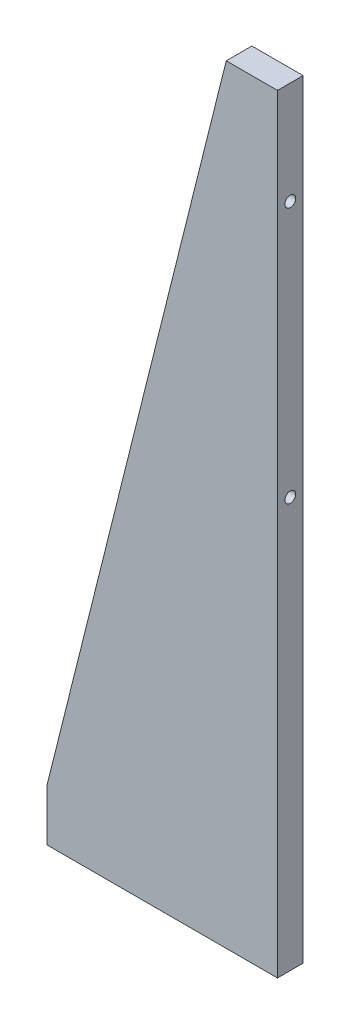
from build123d import *

# Parameters (mm, degrees)
SKETCH_1_W             = 90
SKETCH_1_H             = 300
EXTRUDE_1_DEPTH        = 10
CUT_EXTRUDE_1_REACH    = 158.924
HOLE_WIZARD_M5_1_D     = 4.2
HOLE_WIZARD_M5_1_DEPTH = 14.4
HOLE_WIZARD_M5_1_TIP   = 1.2618073
HOLE_WIZARD_M5_2_D     = 4.2
HOLE_WIZARD_M5_2_DEPTH = 14.4
HOLE_WIZARD_M5_2_TIP   = 1.2618073


with BuildPart() as part:
    # 草图1 → 凸台-拉伸1 (new body)
    with BuildSketch(Plane.XY):
        Rectangle(SKETCH_1_W, SKETCH_1_H)
    extrude(amount=EXTRUDE_1_DEPTH)

    # 草图2 → 切除-拉伸1 (cut, up to next)
    with BuildSketch(Plane.XY.offset(10), mode=Mode.PRIVATE) as cut_extrude_1_sk1:
        Polygon((25, 150), (-45, 150), (-45, -130), align=None)
    cut_extrude_1_tool1 = extrude(cut_extrude_1_sk1.sketch, amount=-CUT_EXTRUDE_1_REACH, mode=Mode.PRIVATE) & part.part
    add(cut_extrude_1_tool1.solids().sort_by_distance((-21.666667, 56.666667, 10))[0], mode=Mode.SUBTRACT)

    # M5 螺纹孔1
    with Locations(Plane(origin=(0, -150, 0), x_dir=(-1, 0, 0), z_dir=(0, -1, 0))):
        with Locations((-25, -5), (25, -5)):
            Hole(HOLE_WIZARD_M5_1_D / 2, depth=HOLE_WIZARD_M5_1_DEPTH)
            with Locations((0, 0, -(HOLE_WIZARD_M5_1_DEPTH + HOLE_WIZARD_M5_1_TIP / 2))):  # 118° drill point
                Cone(0, HOLE_WIZARD_M5_1_D / 2, HOLE_WIZARD_M5_1_TIP, mode=Mode.SUBTRACT)

    # M5 螺纹孔2
    with Locations(Plane(origin=(45, 0, 0), x_dir=(0, 0, -1), z_dir=(1, 0, 0))):
        with Locations((-5, 110), (-5, 10)):
            Hole(HOLE_WIZARD_M5_2_D / 2, depth=HOLE_WIZARD_M5_2_DEPTH)
            with Locations((0, 0, -(HOLE_WIZARD_M5_2_DEPTH + HOLE_WIZARD_M5_2_TIP / 2))):  # 118° drill point
                Cone(0, HOLE_WIZARD_M5_2_D / 2, HOLE_WIZARD_M5_2_TIP, mode=Mode.SUBTRACT)


solid = part.part
